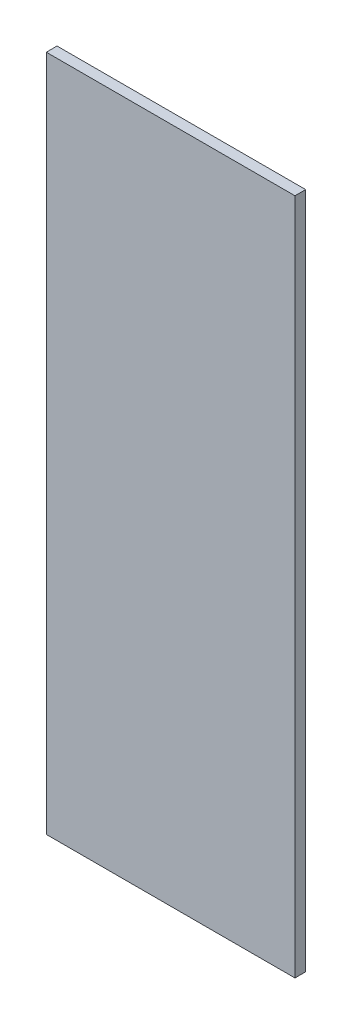
SolidWorks part; units mm, degrees
ref_plane "前视基准面" through (0, 0, 0) normal (0, 0, 1) x (1, 0, 0)
ref_plane "上视基准面" through (0, 0, 0) normal (0, 1, 0) x (1, 0, 0)
ref_plane "右视基准面" through (0, 0, 0) normal (1, 0, 0) x (0, 0, -1)
sketch "草图1" plane through (0, 0, 0) normal (0, 0, 1) x (1, 0, 0)
  line L1 (-410, 910) -> (410, 910)
  line L2 (-410, 910) -> (-410, -910)
  line L3 (-410, -910) -> (410, -910)
  line L4 (410, 910) -> (410, -910)
  line L5 (-410, 910) -> (410, -910) construction
  line L6 (-410, -910) -> (410, 910) construction
  point P0 (0, 0)
  dimension "D1" = 820
  dimension "D2" = 1820
extrude "凸台-拉伸1" add sketch "草图1" along normal blind 25
sketch "草图2" plane through (0, 0, 25) normal (0, 0, 1) x (1, 0, 0)
  line L0 (410, 910) -> (-410, 910) construction
  line L1 (-290, -790) -> (290, -790)
  line L2 (-290, -790) -> (-290, 790)
  line L3 (-290, 790) -> (290, 790)
  line L4 (290, -790) -> (290, 790)
  line L5 (-290, -790) -> (290, 790) construction
  line L6 (-290, 790) -> (290, -790) construction
  line L7 (410, -910) -> (410, 910) construction
  point P0 (0, 0)
  dimension "D1" = 120
  dimension "D2" = 120
extrude "切除-拉伸1" cut sketch "草图2" against normal through all flip side to cut
